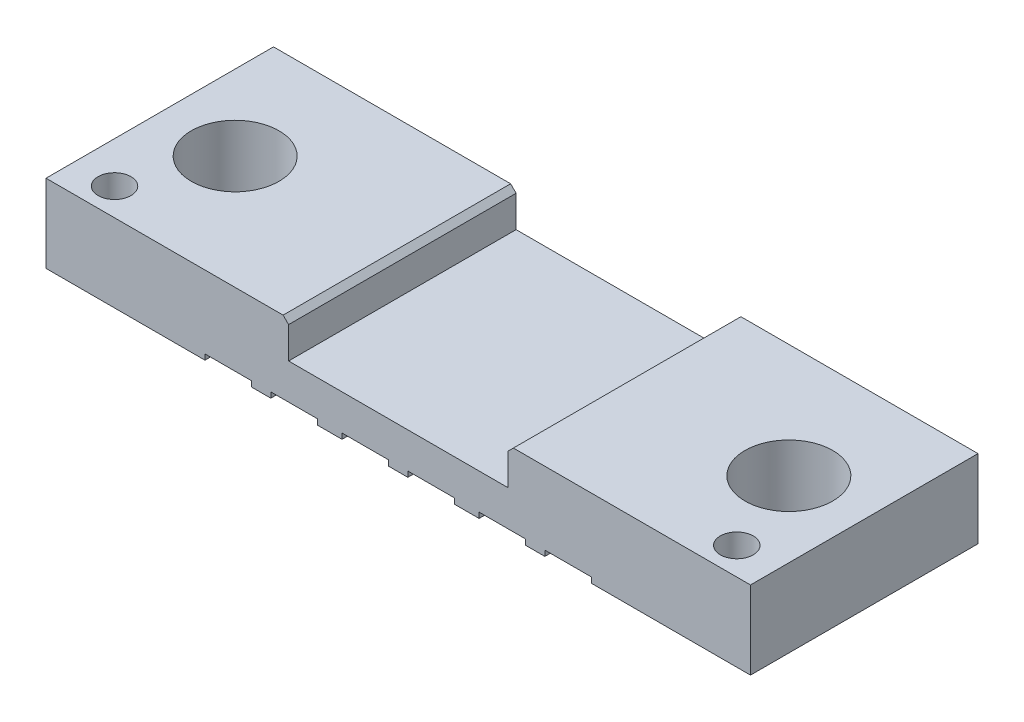
SolidWorks part; units mm, degrees
ref_plane "Front Plane" through (0, 0, 0) normal (0, 0, 1) x (1, 0, 0)
ref_plane "Top Plane" through (0, 0, 0) normal (0, 1, 0) x (1, 0, 0)
ref_plane "Right Plane" through (0, 0, 0) normal (1, 0, 0) x (0, 0, -1)
sketch "Sketch1" plane through (0, 0, 0) normal (0, 1, 0) x (1, 0, 0)
  line L1 (-12.85, 4.15) -> (12.85, 4.15)
  line L2 (-12.85, 4.15) -> (-12.85, -4.15)
  line L3 (-12.85, -4.15) -> (12.85, -4.15)
  line L4 (12.85, 4.15) -> (12.85, -4.15)
  line L5 (-12.85, 4.15) -> (12.85, -4.15) construction
  line L6 (-12.85, -4.15) -> (12.85, 4.15) construction
  point P0 (0, 0)
  dimension "D1" = 25.7
  dimension "D2" = 8.3
extrude "Boss-Extrude1" add sketch "Sketch1" along normal blind 2.85
sketch "Sketch2" plane through (0, 2.85, 0) normal (0, 1, 0) x (1, 0, 0)
  line L0 (0, 0) -> (0, 50000) construction
  line L1 (0, 0) -> (-50000, 0) construction
  line L3 (-12.85, -4.15) -> (12.85, -4.15) construction
  circle A0 centre (-10.1, 0) radius 1.6
  circle A1 centre (-11.35, -3.15) radius 0.6
  circle A2 centre (10.1, 0) radius 1.6
  circle A3 centre (11.35, -3.15) radius 0.6
  dimension "D4" = 22.7
  dimension "D5" = 1.2
  dimension "D6" = 3.2
  dimension "D1" = 20.2
  dimension "D3" = 1
extrude "Cut-Extrude1" cut sketch "Sketch2" against normal through all
sketch "Sketch3" plane through (0, 0, 0) normal (0, -1, 0) x (1, 0, 0)
  line L0 (0, 0) -> (0, -50000) construction
  line L1 (-12.85, 4.15) -> (12.85, 4.15) construction
  line L2 (-7.05, 4.15) -> (-5.35, 4.15)
  line L3 (-7.05, 4.15) -> (-7.05, -4.15)
  line L4 (-7.05, -4.15) -> (-5.35, -4.15)
  line L5 (-5.35, 4.15) -> (-5.35, -4.15)
  line L6 (12.85, -4.15) -> (-12.85, -4.15) construction
  line L7 (0.35, 4.15) -> (0.35, -4.15)
  line L8 (-4.65, 4.15) -> (-2.95, 4.15)
  line L9 (-4.65, 4.15) -> (-4.65, -4.15)
  line L10 (-4.65, -4.15) -> (-2.95, -4.15)
  line L11 (-2.95, 4.15) -> (-2.95, -4.15)
  line L12 (-2.05, 4.15) -> (-0.35, 4.15)
  line L13 (-2.05, 4.15) -> (-2.05, -4.15)
  line L14 (-2.05, -4.15) -> (-0.35, -4.15)
  line L15 (-0.35, 4.15) -> (-0.35, -4.15)
  line L16 (2.05, -4.15) -> (0.35, -4.15)
  line L17 (2.05, 4.15) -> (2.05, -4.15)
  line L18 (2.05, 4.15) -> (0.35, 4.15)
  line L19 (2.95, 4.15) -> (2.95, -4.15)
  line L20 (4.65, -4.15) -> (2.95, -4.15)
  line L21 (4.65, 4.15) -> (4.65, -4.15)
  line L22 (4.65, 4.15) -> (2.95, 4.15)
  line L23 (5.35, 4.15) -> (5.35, -4.15)
  line L24 (7.05, -4.15) -> (5.35, -4.15)
  line L25 (7.05, 4.15) -> (7.05, -4.15)
  line L26 (7.05, 4.15) -> (5.35, 4.15)
  dimension "D1" = 1.7
  dimension "D2" = 0.7
  dimension "D3" = 1.7
  dimension "D4" = 5.9
  dimension "D5" = 1.7
  dimension "D6" = 10.7
extrude "Cut-Extrude2" cut sketch "Sketch3" against normal blind 0.2
sketch "Sketch4" plane through (0, 2.85, 0) normal (0, 1, 0) x (1, 0, 0)
  line L0 (-12.85, -4.15) -> (12.85, -4.15) construction
  line L1 (-4, 4.15) -> (4, 4.15)
  line L2 (-4, 4.15) -> (-4, -4.15)
  line L3 (-4, -4.15) -> (4, -4.15)
  line L4 (4, 4.15) -> (4, -4.15)
  line L5 (-4, 4.15) -> (4, -4.15) construction
  line L6 (-4, -4.15) -> (4, 4.15) construction
  point P0 (0, 0)
  dimension "D1" = 8
extrude "Cut-Extrude3" cut sketch "Sketch4" against normal blind 1.35
chamfer "Chamfer1" distance 0.2 angle 45 2 edges at (4, 2.85, 0) (-4, 2.85, 0)
